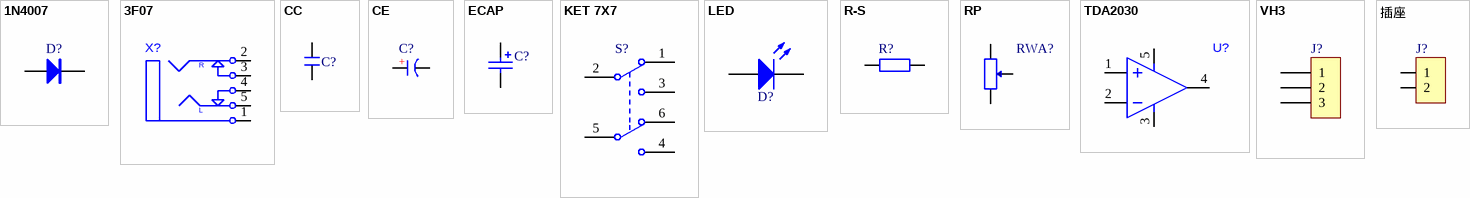
[diagram p0: symbols 1N4007 to 插座]
# Altium schematic symbol library MISC82779-10.SCHLIB: 12 symbols
Pins are listed as number, name and electrical type; pins without a type are passive.


## 1N4007
designator D?
rectifier diode
footprint DO-41 (2.6*9.1mm (diameter, lead pitch))
footprint SOD-123 (2.7x1.6x1.1mm (L x W x H, excluding leads))
footprint SMA (4.5x2.6*2.2mm (L x W x H, excluding leads))
footprint DO-41V (2.6*3.5mm (diameter, lead pitch))
pins: 1 A, 2 K

## 3F07
designator X?
footprint 3F07
pins: 1, 2, 3, 4, 5

## CC
designator C?
ceramic disc capacitor
footprint CC 2.2*5 (Lead pitch 2.2mm, diameter 5mm)
pins: 1, 2

## CE
designator C?
through-hole electrolytic capacitor
footprint CAP 1.5*4*8 (Lead pitch 1.5mm, diameter 4mm, height 8mm)
footprint CAP 1.5*4*8 - BK (Lead pitch 1.5mm, diameter 4mm, height 8mm)
footprint CAP 1.5*4*8 - GD (Lead pitch 1.5mm, diameter 4mm, height 8mm)
footprint CAP 1.5*4*8-H (Lead pitch 1.5mm, diameter 4mm, height 8mm)
footprint CAP 1.5*4*8-H - BK (Lead pitch 1.5mm, diameter 4mm, height 8mm)
footprint CAP 1.5*4*8-H - GD (Lead pitch 1.5mm, diameter 4mm, height 8mm)
footprint CAP 2.0*5*11 (Lead pitch 2mm, diameter 5mm, height 11mm)
footprint CAP 2.0*5*11 - BK (Lead pitch 2mm, diameter 5mm, height 11mm)
footprint CAP 2.0*5*11 - GD (Lead pitch 2mm, diameter 5mm, height 11mm)
footprint CAP 2.0*5*11-H (Lead pitch 2mm, diameter 5mm, height 11mm)
footprint CAP 2.0*5*11-H - BK (Lead pitch 2mm, diameter 5mm, height 11mm)
footprint CAP 2.0*5*11-H - GD (Lead pitch 2mm, diameter 5mm, height 11mm)
footprint CAP 2.5*5*11 (Lead pitch 2.5mm, diameter 5mm, height 11mm)
footprint CAP 2.5*5*11 - BK (Lead pitch 2.5mm, diameter 5mm, height 11mm)
footprint CAP 2.5*5*11 - GD (Lead pitch 2.5mm, diameter 5mm, height 11mm)
footprint CAP 2.5*5*11-H (Lead pitch 2.5mm, diameter 5mm, height 11mm)
footprint CAP 2.5*5*11-H - BK (Lead pitch 2.5mm, diameter 5mm, height 11mm)
footprint CAP 2.5*5*11-H - GD (Lead pitch 2.5mm, diameter 5mm, height 11mm)
footprint CAP 2.5*6.3*7 (Lead pitch 2.5mm, diameter 6.3mm, height 7mm)
footprint CAP 2.5*6.3*7 - BK (Lead pitch 2.5mm, diameter 6.3mm, height 7mm)
footprint CAP 2.5*6.3*7 - GD (Lead pitch 2.5mm, diameter 6.3mm, height 7mm)
footprint CAP 2.5*6.3*7-H (Lead pitch 2.5mm, diameter 6.3mm, height 7mm)
footprint CAP 2.5*6.3*7-H - BK (Lead pitch 2.5mm, diameter 6.3mm, height 7mm)
footprint CAP 2.5*6.3*7-H - GD (Lead pitch 2.5mm, diameter 6.3mm, height 7mm)
footprint CAP 2.5*6.3*11.2 (Lead pitch 2.5mm, diameter 6.3mm, height 11.2mm)
footprint CAP 2.5*6.3*11.2 - BK (Lead pitch 2.5mm, diameter 6.3mm, height 11.2mm)
footprint CAP 2.5*6.3*11.2 - GD (Lead pitch 2.5mm, diameter 6.3mm, height 11.2mm)
footprint CAP 2.5*6.3*11.2-H (Lead pitch 2.5mm, diameter 6.3mm, height 11.2mm)
footprint CAP 2.5*6.3*11.2-H - BK (Lead pitch 2.5mm, diameter 6.3mm, height 11.2mm)
footprint CAP 2.5*6.3*11.2-H - GD (Lead pitch 2.5mm, diameter 6.3mm, height 11.2mm)
footprint CAP 3.5*8*11.5 (Lead pitch 3.5mm, diameter 8mm, height 11.5mm)
footprint CAP 3.5*8*11.5 - BK (Lead pitch 3.5mm, diameter 8mm, height 11.5mm)
footprint CAP 3.5*8*11.5 - GD (Lead pitch 3.5mm, diameter 8mm, height 11.5mm)
footprint CAP 3.5*8*11.5-H (Lead pitch 3.5mm, diameter 8mm, height 11.5mm)
footprint CAP 3.5*8*11.5-H - BK (Lead pitch 3.5mm, diameter 8mm, height 11.5mm)
footprint CAP 3.5*8*11.5-H - GD (Lead pitch 3.5mm, diameter 8mm, height 11.5mm)
footprint CAP 5.0*10*12.5 (Lead pitch 5mm, diameter 10mm, height 12.5mm)
footprint CAP 5.0*10*12.5 - BK (Lead pitch 5mm, diameter 10mm, height 12.5mm)
footprint CAP 5.0*10*12.5 - GD (Lead pitch 5mm, diameter 10mm, height 12.5mm)
footprint CAP 5.0*10*12.5-H (Lead pitch 5mm, diameter 10mm, height 12.5mm)
footprint CAP 5.0*10*12.5-H - BK (Lead pitch 5mm, diameter 10mm, height 12.5mm)
footprint CAP 5.0*10*12.5-H - GD (Lead pitch 5mm, diameter 10mm, height 12.5mm)
footprint CAP 5.0*10*16 (Lead pitch 5mm, diameter 10mm, height 16mm)
footprint CAP 5.0*10*16 - BK (Lead pitch 5mm, diameter 10mm, height 16mm)
footprint CAP 5.0*10*16 - GD (Lead pitch 5mm, diameter 10mm, height 16mm)
footprint CAP 5.0*10*16-H (Lead pitch 5mm, diameter 10mm, height 16mm)
footprint CAP 5.0*10*16-H - BK (Lead pitch 5mm, diameter 10mm, height 16mm)
footprint CAP 5.0*10*16-H - GD (Lead pitch 5mm, diameter 10mm, height 16mm)
footprint CAP 5.0*10*20 (Lead pitch 5mm, diameter 10mm, height 20mm)
footprint CAP 5.0*10*20 - BK (Lead pitch 5mm, diameter 10mm, height 20mm)
footprint CAP 5.0*10*20 - GD (Lead pitch 5mm, diameter 10mm, height 20mm)
footprint CAP 5.0*10*20-H (Lead pitch 5mm, diameter 10mm, height 20mm)
footprint CAP 5.0*10*20-H - BK (Lead pitch 5mm, diameter 10mm, height 20mm)
footprint CAP 5.0*10*20-H - GD (Lead pitch 5mm, diameter 10mm, height 20mm)
footprint CAP 5.0*12.5*20 (Lead pitch 5mm, diameter 12.5mm, height 20mm)
footprint CAP 5.0*12.5*20 - BK (Lead pitch 5mm, diameter 12.5mm, height 20mm)
footprint CAP 5.0*12.5*20 - GD (Lead pitch 5mm, diameter 12.5mm, height 20mm)
footprint CAP 5.0*12.5*20-H (Lead pitch 5mm, diameter 12.5mm, height 20mm)
footprint CAP 5.0*12.5*20-H - BK (Lead pitch 5mm, diameter 12.5mm, height 20mm)
footprint CAP 5.0*12.5*20-H - GD (Lead pitch 5mm, diameter 12.5mm, height 20mm)
footprint CAP 5.0*12.5*25 (Lead pitch 5mm, diameter 12.5mm, height 25mm)
footprint CAP 5.0*12.5*25 - BK (Lead pitch 5mm, diameter 12.5mm, height 25mm)
footprint CAP 5.0*12.5*25 - GD (Lead pitch 5mm, diameter 12.5mm, height 25mm)
footprint CAP 5.0*12.5*25-H (Lead pitch 5mm, diameter 12.5mm, height 25mm)
footprint CAP 5.0*12.5*25-H - BK (Lead pitch 5mm, diameter 12.5mm, height 25mm)
footprint CAP 5.0*12.5*25-H - GD (Lead pitch 5mm, diameter 12.5mm, height 25mm)
footprint CAP 7.5*16*25 (Lead pitch 7.5mm, diameter 16mm, height 25mm)
footprint CAP 7.5*16*25 - BK (Lead pitch 7.5mm, diameter 16mm, height 25mm)
footprint CAP 7.5*16*25 - GD (Lead pitch 7.5mm, diameter 16mm, height 25mm)
footprint CAP 7.5*16*25-H (Lead pitch 7.5mm, diameter 16mm, height 25mm)
footprint CAP 7.5*16*25-H - BK (Lead pitch 7.5mm, diameter 16mm, height 25mm)
footprint CAP 7.5*16*25-H - GD (Lead pitch 7.5mm, diameter 16mm, height 25mm)
footprint CAP 7.5*16*31.5 (Lead pitch 7.5mm, diameter 16mm, height 31.5mm)
footprint CAP 7.5*16*31.5 - BK (Lead pitch 7.5mm, diameter 16mm, height 31.5mm)
footprint CAP 7.5*16*31.5 - GD (Lead pitch 7.5mm, diameter 16mm, height 31.5mm)
footprint CAP 7.5*16*31.5-H (Lead pitch 7.5mm, diameter 16mm, height 31.5mm)
footprint CAP 7.5*16*31.5-H - BK (Lead pitch 7.5mm, diameter 16mm, height 31.5mm)
footprint CAP 7.5*16*31.5-H - GD (Lead pitch 7.5mm, diameter 16mm, height 31.5mm)
footprint CAP 7.5*18*35.5 (Lead pitch 7.5mm, diameter 18mm, height 35.5mm)
footprint CAP 7.5*18*35.5 - BK (Lead pitch 7.5mm, diameter 18mm, height 35.5mm)
footprint CAP 7.5*18*35.5 - GD (Lead pitch 7.5mm, diameter 18mm, height 35.5mm)
footprint CAP 7.5*18*35.5-H (Lead pitch 7.5mm, diameter 18mm, height 35.5mm)
footprint CAP 7.5*18*35.5-H - BK (Lead pitch 7.5mm, diameter 18mm, height 35.5mm)
footprint CAP 7.5*18*35.5-H - GD (Lead pitch 7.5mm, diameter 18mm, height 35.5mm)
footprint CAP 10*22*31.5 (Lead pitch 10mm, diameter 22mm, height 31.5mm)
footprint CAP 10*22*31.5 - BK (Lead pitch 10mm, diameter 22mm, height 31.5mm)
footprint CAP 10*22*31.5 - GD (Lead pitch 10mm, diameter 22mm, height 31.5mm)
footprint CAP 10*22*40 (Lead pitch 10mm, diameter 22mm, height 40mm)
footprint CAP 10*22*40 - BK (Lead pitch 10mm, diameter 22mm, height 40mm)
footprint CAP 10*22*40 - GD (Lead pitch 10mm, diameter 22mm, height 40mm)
pins: 1 A, 2 K

## ECAP
designator C?
footprint EC100
pins: 1, 2

## KET 7X7
designator S?
7*7 self-locking switch
footprint KFT DIP-7X7 (Self-locking switch, spec: 7*7mm)
pins: 1 NC1, 2 COM2, 3 NO1, 4 NO2, 5 COM2, 6 NC2

## LED
designator D?
LED
footprint LED 5MM-W (White 5mm through-hole LED)
pins: 1 A, 2 K

## R-S
designator R?
color-band resistor
footprint RS 1/2W (Through-hole color-band resistor, lead pitch 12.5mm, diameter 3mm)
footprint RS 1/2W-V4 (Through-hole color-band resistor, lead pitch 4mm, diameter 3mm)
footprint RS 1/4W (Through-hole color-band resistor, lead pitch 9mm, diameter 2.3mm)
footprint RS 1/4W-V3 (Through-hole color-band resistor, lead pitch 3mm, diameter 2.3mm)
footprint RS 1/8W (Through-hole color-band resistor, lead pitch 6mm, diameter 1.5mm)
footprint RS 1/8W-V2 (Through-hole color-band resistor, lead pitch 2mm, diameter 1.5mm)
footprint RS 1W (Through-hole color-band resistor, lead pitch 15mm, diameter 4mm)
footprint RS 1W-F5 (Through-hole color-band resistor, lead pitch 15mm, diameter 4mm, standoff 5mm)
footprint RS 1W-V5 (Through-hole color-band resistor, lead pitch 5mm, diameter 4mm)
footprint RS 2W (Through-hole color-band resistor, lead pitch 20mm, diameter 5mm)
footprint RS 2W-F5 (Through-hole color-band resistor, lead pitch 20mm, diameter 5mm, standoff 5mm)
footprint RS 2W-V6 (Through-hole color-band resistor, lead pitch 6mm, diameter 5mm)
footprint RS 3W (Through-hole color-band resistor, lead pitch 25mm, diameter 6mm)
footprint RS 3W-F5 (Through-hole color-band resistor, lead pitch 25mm, diameter 6mm, standoff 5mm)
footprint RS 3W-V7 (Through-hole color-band resistor, lead pitch 7mm, diameter 6mm)
footprint RS 5W (Through-hole color-band resistor, lead pitch 30mm, diameter 8mm)
footprint RS 5W-F5 (Through-hole color-band resistor, lead pitch 30mm, diameter 8mm, standoff 5mm)
footprint RS 5W-V8 (Through-hole color-band resistor, lead pitch 8mm, diameter 8mm)
pins: 1, 2

## RP
designator RWA?
single-gang potentiometer
footprint 3296W (Precise Multi-Winding Adjustable Resistor)
footprint 3306W
footprint 3319P
footprint 3362P
footprint 3386W
footprint RM065 (Blue-white adjustable potentiometer)
footprint WH148-1-G15 (Single-gang potentiometer, lead pitch: 5mm, shaft length: 15mm)
footprint WH148-1-G18 (Single-gang potentiometer, lead pitch: 5mm, shaft length: 18mm)
footprint WH148-1-G20 (Single-gang potentiometer, lead pitch: 5mm, shaft length: 20mm)
footprint WH148-1-G25 (Single-gang potentiometer, lead pitch: 5mm, shaft length: 25mm)
footprint 3266W (L: 7mm, W: 4.8mm, H: 7.5mm)
footprint 3266X (L: 7mm, W: 4.8mm, H: 7.5mm)
footprint 3266Y (L: 7mm, W: 4.8mm, H: 7.5mm)
footprint 3266Z (L: 7mm, W: 4.8mm, H: 7.5mm)
footprint XV09223NPV-20F (L 9.85mm, W 11.55mm, H 20mm)
footprint XV09223NPV-25F (L 9.85mm, W 11.55mm, H 25mm)
footprint XV09223NPV-30F (L 9.85mm, W 11.55mm, H 30mm)
footprint 3006P (19.05mm*4.83mm*6.35mm (L*W*H))
pins: 1, 2, 3

## TDA2030
designator U?
footprint TDA2030
pins: 1, 2, 3, 4, 5

## VH3
designator J?
footprint VH3.96-3A
footprint VH3.96-3AW
footprint VH3.96-3AWD
pins: 1, 2, 3

## 插座
designator J?
footprint DZ
pins: 1, 2